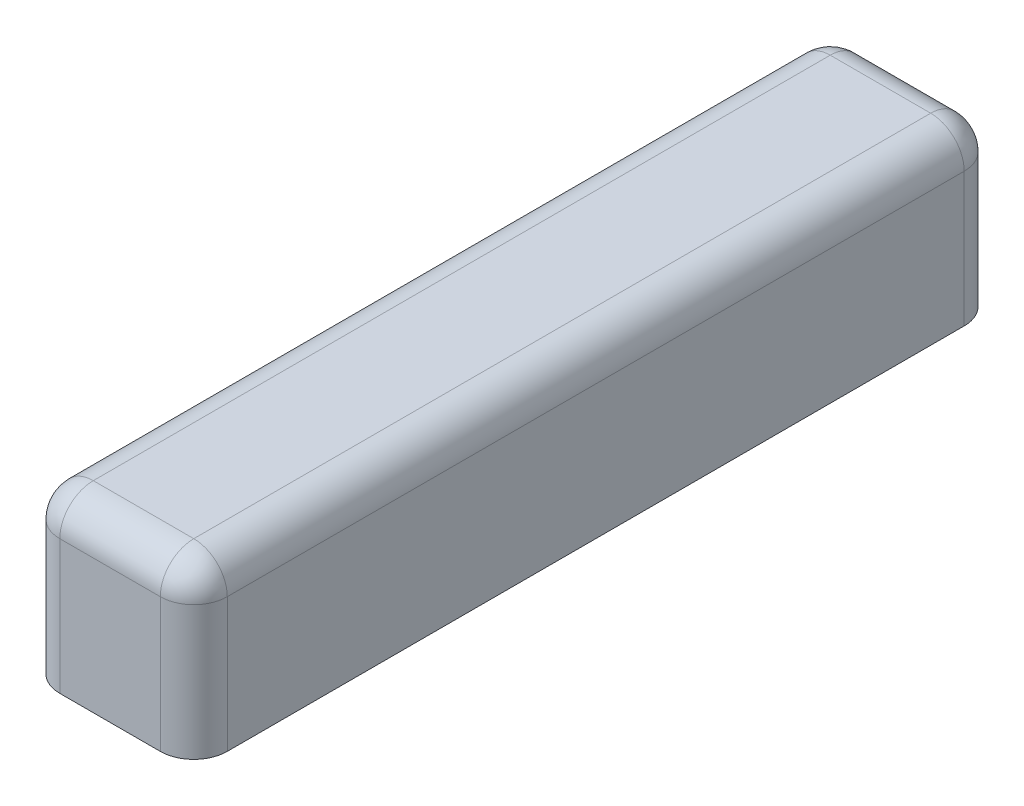
from build123d import *

# Parameters (mm, degrees)
SKETCH_1_W          = 50
SKETCH_1_H          = 50
EXTRUDE_2_DEPTH     = 240
EXTRUDE_3_DEPTH     = 5
FILLET_1_R          = 10
SKETCH_3_W          = 340
SKETCH_3_H          = 5
CUT_EXTRUDE_1_DEPTH = 59


with BuildPart() as part:
    # 草图1 → 凸台-拉伸2 (new body)
    with BuildSketch(Plane.XY):
        with Locations((25, 25)):
            Rectangle(SKETCH_1_W, SKETCH_1_H)
    extrude(amount=EXTRUDE_2_DEPTH)

    # 草图2 → 凸台-拉伸3 (add)
    with BuildSketch(Plane.XZ):
        Polygon((0, 240), (0, 290), (50, 290), (50, 0), (50, -50), (0, -50), align=None)
    extrude(amount=EXTRUDE_3_DEPTH)

    # 圆角1
    fillet_1_edges = [part.edges().sort_by_distance(p)[0] for p in [
        (25, 50, 240),
        (0, 25, 240),
        (50, 25, 240),
        (50, 50, 120),
        (50, 25, 0),
        (0, 25, 0),
        (25, 50, 0),
        (0, 50, 120),
    ]]
    fillet(fillet_1_edges, radius=FILLET_1_R)

    # 草图3 → 切除-拉伸1 (cut)
    with BuildSketch(Plane.ZY):
        with Locations((120, -2.5)):
            Rectangle(SKETCH_3_W, SKETCH_3_H)
    extrude(amount=-CUT_EXTRUDE_1_DEPTH, mode=Mode.SUBTRACT)


solid = part.part
